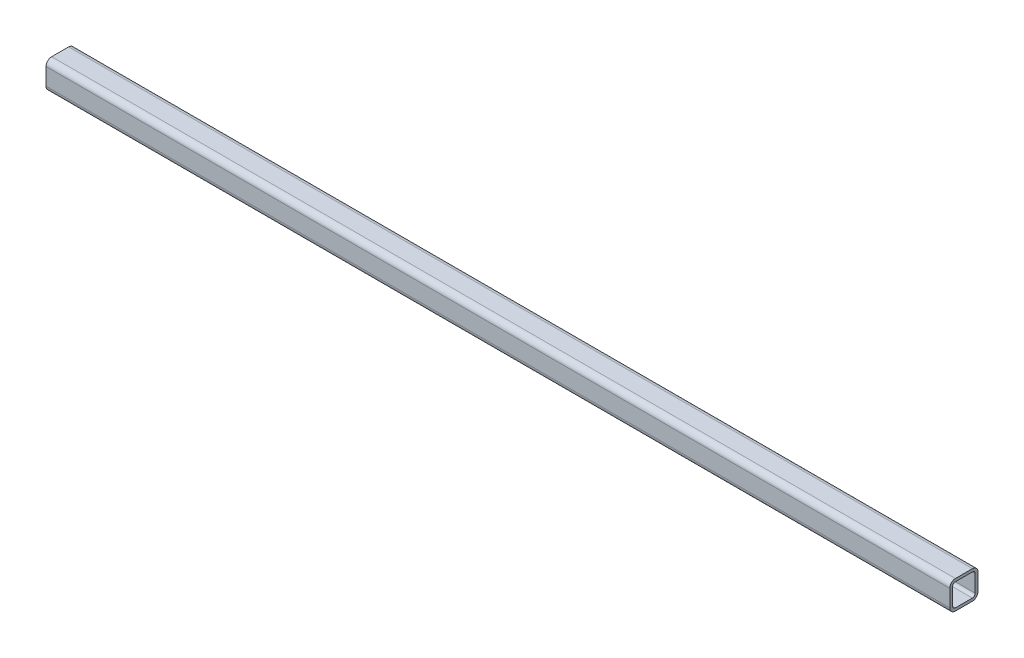
SolidWorks part; units mm, degrees
material "普通碳钢"
ref_plane "Front Plane" through (0, 0, 0) normal (0, 0, 1) x (1, 0, 0)
ref_plane "Top Plane" through (0, 0, 0) normal (0, 1, 0) x (1, 0, 0)
ref_plane "Right Plane" through (0, 0, 0) normal (1, 0, 0) x (0, 0, -1)
sketch "草图1" plane through (0, 0, 0) normal (0, 0, 1) x (1, 0, 0)
  line L0 (-1000, 0) -> (280, 0)
  dimension "D1" = 1280
  dimension "D2" = 1000
other "Square Tube 40 X 40 X 4(1)"
ref_plane "Plane1" through (-1000, 0, 0) normal (1, 0, 0) x (0, 1, 0)
sketch "Sketch1" plane through (-1000, 0, 0) normal (1, 0, 0) x (0, 1, 0)
  line L0 (-12, -16) -> (12, -16)
  line L1 (-16, -12) -> (-16, 12)
  line L2 (12, 16) -> (-12, 16)
  line L3 (16, 12) -> (16, -12)
  line L4 (-12, -20) -> (12, -20)
  line L5 (-20, -12) -> (-20, 12)
  line L6 (12, 20) -> (-12, 20)
  line L7 (20, 12) -> (20, -12)
  arc A0 (20, 12) -> (12, 20) centre (12, 12) ccw
  arc A1 (12, -20) -> (20, -12) centre (12, -12) ccw
  arc A2 (-20, -12) -> (-12, -20) centre (-12, -12) ccw
  arc A3 (-12, 20) -> (-20, 12) centre (-12, 12) ccw
  arc A4 (-12, 16) -> (-16, 12) centre (-12, 12) ccw
  arc A5 (16, 12) -> (12, 16) centre (12, 12) ccw
  arc A6 (12, -16) -> (16, -12) centre (12, -12) ccw
  arc A7 (-16, -12) -> (-12, -16) centre (-12, -12) ccw
  point P0 (-20, 0)
  point P1 (20, 0)
  point P2 (0, 20)
  point P3 (0, -20)
  point P4 (0, 0)
  point P5 (-20, -20)
  point P6 (20, -20)
  point P7 (20, 20)
  point P8 (-20, 20)
  point P33 (0, 0)
  dimension "D1" = 8
  dimension "Thickness" = 4
  dimension "V_leg" = 40
